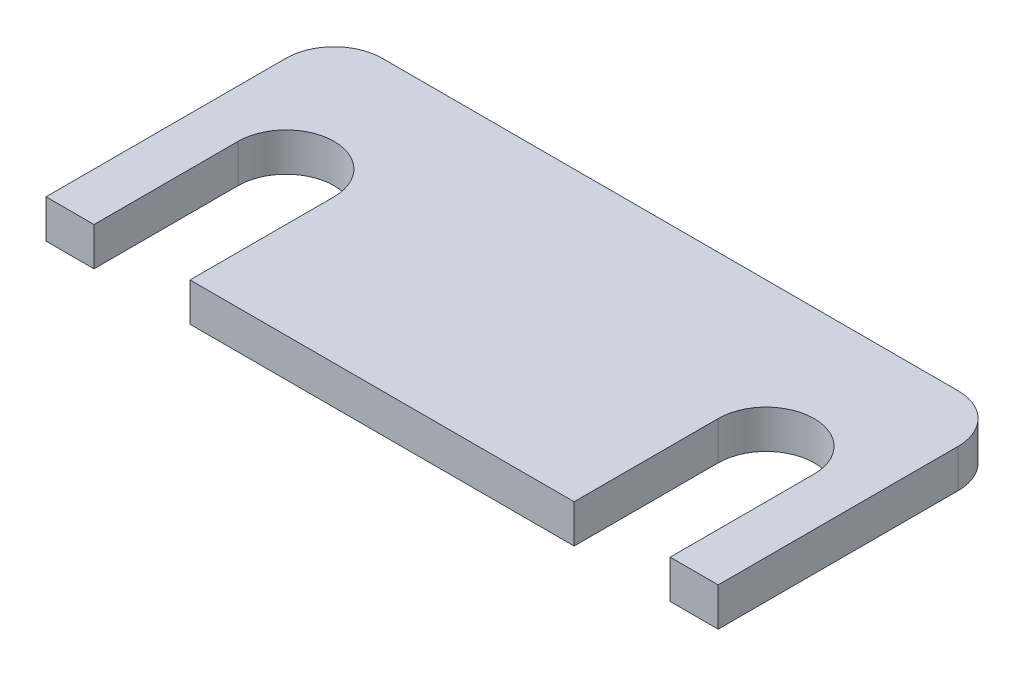
from build123d import *

# Parameters (mm, degrees)
EXTRUDE_1_DEPTH = 4


with BuildPart() as part:
    # 草图1 → 凸台-拉伸1 (new body)
    with BuildSketch(Plane(origin=(0, 0, 0), x_dir=(1, 0, 0), z_dir=(0, 1, 0))):
        with BuildLine():
            Line((30, 30), (-30, 30))
            ThreePointArc((-30, 30), (-33.535533906, 28.535533906), (-35, 25))
            Line((-35, 25), (-35, 0))
            Line((-35, 0), (-30, 0))
            Line((-30, 0), (-30, 15))
            ThreePointArc((-30, 15), (-25, 20), (-20, 15))
            Line((-20, 15), (-20, 0))
            Line((-20, 0), (20, 0))
            Line((20, 0), (20, 15))
            ThreePointArc((20, 15), (25, 20), (30, 15))
            Line((30, 15), (30, 0))
            Line((30, 0), (35, 0))
            Line((35, 0), (35, 25))
            ThreePointArc((35, 25), (33.535533906, 28.535533906), (30, 30))
        make_face()
    extrude(amount=EXTRUDE_1_DEPTH)


solid = part.part
